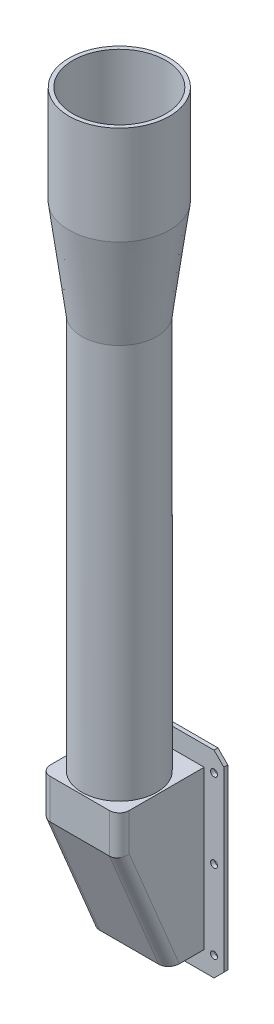
from build123d import *

# Parameters (mm, degrees)
SKETCH1_W               = 40
SKETCH1_H               = 80
BOSS_EXTRUDE1_DEPTH     = 45
SKETCH2_R               = 19
BOSS_EXTRUDE2_DEPTH     = 200
CUT_EXTRUDE1_DEPTH      = 248.436860633
CUT_EXTRUDE1_DEPTH_BACK = 248.436860633
SHELL1_T                = -2
SKETCH4_W               = 60
SKETCH4_H               = 100
SKETCH4_W_2             = 40
SKETCH4_H_2             = 80
BOSS_EXTRUDE3_DEPTH     = 2
CHAMFER1_SIZE           = 5
SKETCH5_R               = 1.75
CUT_EXTRUDE2_DEPTH      = 10
SKETCH6_R               = 1.75
CUT_EXTRUDE3_DEPTH      = 10
FILLET1_R               = 5


with BuildPart() as part:
    # Sketch1 → Boss-Extrude1 (new body)
    with BuildSketch(Plane.XY):
        Rectangle(SKETCH1_W, SKETCH1_H)
    extrude(amount=BOSS_EXTRUDE1_DEPTH)

    # Sketch2 → Boss-Extrude2 (add)
    with BuildSketch(Plane(origin=(0, 40, 0), x_dir=(1, 0, 0), z_dir=(0, 1, 0))):
        with Locations(Location((0, -25, 0), (0, 0, 90))):
            Circle(SKETCH2_R)
    extrude(amount=BOSS_EXTRUDE2_DEPTH)

    # Sketch3 → Cut-Extrude1 (cut, two sides: drawn at the far end of the back side and taken through both)
    with BuildSketch(Plane(origin=(20, 0, 0), x_dir=(0, 0, -1), z_dir=(1, 0, 0)).offset(-CUT_EXTRUDE1_DEPTH_BACK)):
        Polygon((200.08758149, -568.210195577), (-20, -40), (-45, 20), (-265.08758149, 548.210195577), (-1321.507972644, 108.035032596), (-856.332809663, -1008.385358557), align=None)
    extrude(amount=CUT_EXTRUDE1_DEPTH + CUT_EXTRUDE1_DEPTH_BACK, mode=Mode.SUBTRACT)

    # Shell1
    shell1_openings = [part.faces().sort_by_distance(p)[0] for p in [
        (0, 240, 25),
        (0, 0, 0),
    ]]
    offset(amount=SHELL1_T, openings=shell1_openings, kind=Kind.INTERSECTION)

    # Sketch4 → Boss-Extrude3 (add)
    with BuildSketch(Plane(origin=(0, 0, 0), x_dir=(-1, 0, 0), z_dir=(0, 0, -1))):
        Rectangle(SKETCH4_W, SKETCH4_H)
        Rectangle(SKETCH4_W_2, SKETCH4_H_2, mode=Mode.SUBTRACT)
    extrude(amount=-BOSS_EXTRUDE3_DEPTH)

    # Chamfer1
    chamfer1_edges = [part.edges().sort_by_distance(p)[0] for p in [
        (-30, -50, 1),
        (30, -50, 1),
        (30, 50, 1),
        (-30, 50, 1),
    ]]
    chamfer(chamfer1_edges, length=CHAMFER1_SIZE)

    # Sketch5 → Cut-Extrude2 (cut)
    with BuildSketch(Plane.XY.offset(2)):
        with Locations((-25, 0)):
            Circle(SKETCH5_R)
        with Locations((-25, 40)):
            Circle(SKETCH5_R)
        with Locations((-25, -40)):
            Circle(SKETCH5_R)
    cut_extrude2 = extrude(amount=-CUT_EXTRUDE2_DEPTH, mode=Mode.SUBTRACT)

    # Mirror1: Cut-Extrude2 across plane
    add(cut_extrude2.mirror(Plane(origin=(0, 0, 0), x_dir=(0, 0, 1), z_dir=(1, 0, 0))), mode=Mode.SUBTRACT)

    # Sketch6 → Cut-Extrude3 (cut)
    with BuildSketch(Plane.XY.offset(2)):
        with Locations((0, -45)):
            Circle(SKETCH6_R)
    extrude(amount=-CUT_EXTRUDE3_DEPTH, mode=Mode.SUBTRACT)

    # Sketch7 → Revolve1 (revolve)
    with BuildSketch(Plane(origin=(0, 0, 0), x_dir=(0, 0, -1), z_dir=(1, 0, 0))):
        Polygon((-44, 240), (-50.5, 290), (-50.5, 340), (-48.5, 340), (-48.5, 290.129455343), (-41.983170805, 240), align=None)
    revolve(axis=Axis((0, 340, 25), (0, -1, 0)))

    # Fillet1
    fillet1_edges = [part.edges().sort_by_distance(p)[0] for p in [
        (-20, 30, 45),
        (20, 30, 45),
        (20, -10, 32.5),
        (-20, -10, 32.5),
    ]]
    fillet(fillet1_edges, radius=FILLET1_R)


solid = part.part
